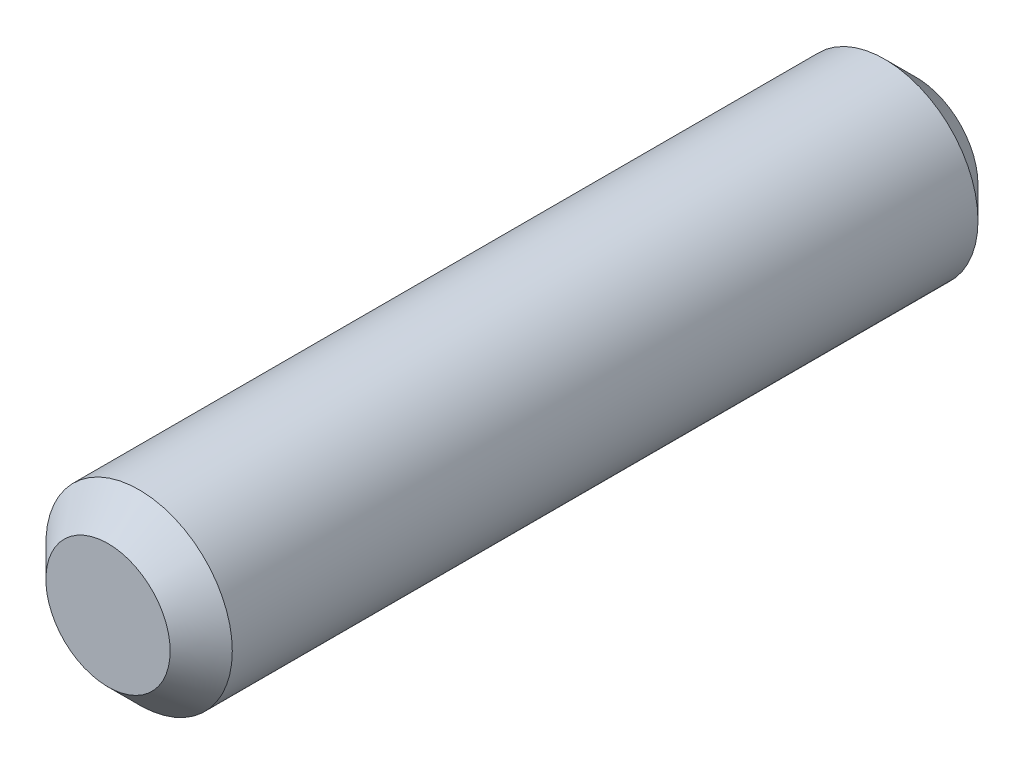
from build123d import *

# Parameters (mm, degrees)
SKETCH_1_R      = 1.5
EXTRUDE_1_DEPTH = 13
CHAMFER_1_SIZE  = 0.5


with BuildPart() as part:
    # 草图1 → 凸台-拉伸1 (new body)
    with BuildSketch(Plane.XY):
        with Locations((-185.609004659, 197.47870093)):
            Circle(SKETCH_1_R)
    extrude(amount=-EXTRUDE_1_DEPTH)

    # 倒角1
    chamfer_1_edges = [part.edges().sort_by_distance(p)[0] for p in [
        (-187.109004659, 197.47870093, 0),
        (-187.109004659, 197.47870093, -13),
    ]]
    chamfer(chamfer_1_edges, length=CHAMFER_1_SIZE)


solid = part.part
